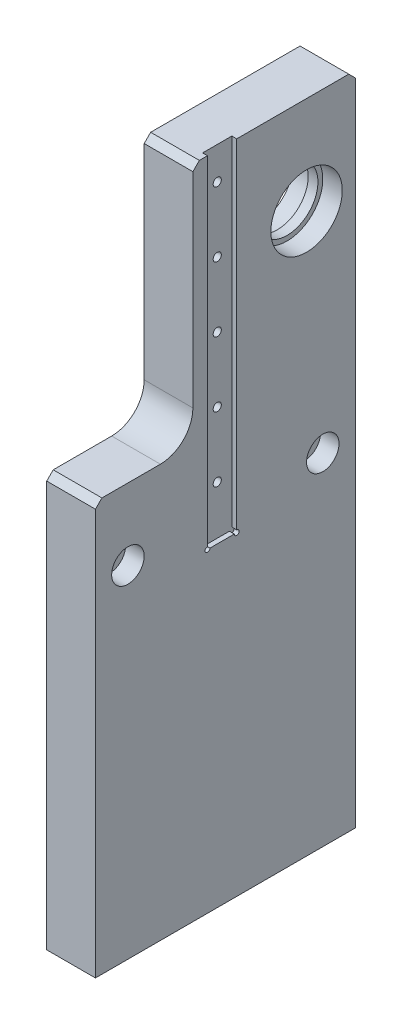
from build123d import *

# Parameters (mm, degrees)
EXTRUDE_1_DEPTH           = 7.5
SKETCH_2_R                = 11
CUT_EXTRUDE_1_DEPTH       = 6
CUT_EXTRUDE_2_REACH       = 111.663
SKETCH_3_R                = 9.5
CUT_EXTRUDE_3_DEPTH       = 1.5
HOLE_WIZARD_M5_1_D        = 4.2
HOLE_WIZARD_M5_1_DEPTH    = 12.4
HOLE_WIZARD_M5_1_TIP      = 1.2618073
HOLE_WIZARD_1_D           = 5.5
HOLE_WIZARD_1_CBORE_D     = 10
HOLE_WIZARD_1_CBORE_DEPTH = 5.7
HOLE_WIZARD_M3_2_D        = 2.5
CUT_EXTRUDE_START         = -6
SKETCH_17_R               = 11
CUT_EXTRUDE_4_DEPTH       = 6
HOLE_WIZARD_M6_1_D        = 5
HOLE_WIZARD_M6_1_DEPTH    = 15
HOLE_WIZARD_M6_1_TIP      = 1.502151548
CHAMFER_1_SIZE            = 2


with BuildPart() as part:
    # 草图1 → 凸台-拉伸1 (new, symmetric)
    with BuildSketch(Plane(origin=(0, 0, 0), x_dir=(0, 0, -1), z_dir=(1, 0, 0))):
        with BuildLine():
            Line((-10, 101), (-10, 36))
            ThreePointArc((-10, 36), (-12.928932188, 28.928932188), (-20, 26))
            Line((-20, 26), (-40, 26))
            Line((-40, 26), (-40, -101))
            Line((-40, -101), (40, -101))
            Line((40, -101), (40, 101))
            Line((40, 101), (-10, 101))
        make_face()
    extrude(amount=EXTRUDE_1_DEPTH, both=True)

    # 草图2 → 切除-拉伸1 (cut)
    with BuildSketch(Plane.ZY.offset(-7.5)):
        with Locations((-25, 71)):
            Circle(SKETCH_2_R)
    extrude(amount=CUT_EXTRUDE_1_DEPTH, mode=Mode.SUBTRACT)

    # 草图3 → 切除-拉伸2 (cut, up to next)
    with BuildSketch(Plane(origin=(-7.5, 0, 0), x_dir=(0, 0, -1), z_dir=(1, 0, 0)), mode=Mode.PRIVATE) as cut_extrude_2_sk1:
        with Locations(Location((25, 71, 0), (0, 0, 180))):
            Circle(SKETCH_3_R)
    cut_extrude_2_tool1 = extrude(cut_extrude_2_sk1.sketch, amount=CUT_EXTRUDE_2_REACH, mode=Mode.PRIVATE) & part.part
    add(cut_extrude_2_tool1.solids().sort_by_distance((-7.5, 71, -25))[0], mode=Mode.SUBTRACT)

    # 草图6 → 切除-拉伸3 (cut)
    with BuildSketch(Plane(origin=(7.5, 0, 0), x_dir=(0, 0, -1), z_dir=(1, 0, 0))):
        with BuildLine():
            Line((-5.5, 101), (3.5, 101))
            Line((3.5, 101), (3.5, -3.25))
            ThreePointArc((3.5, -3.25), (4.030330086, -4.530330086), (2.75, -4))
            Line((2.75, -4), (-4.75, -4))
            ThreePointArc((-4.75, -4), (-6.030330086, -4.530330086), (-5.5, -3.25))
            Line((-5.5, -3.25), (-5.5, 101))
        make_face()
    extrude(amount=-CUT_EXTRUDE_3_DEPTH, mode=Mode.SUBTRACT)

    # M5 螺纹孔1
    with Locations(Plane(origin=(0, -101, 0), x_dir=(-1, 0, 0), z_dir=(0, -1, 0))):
        with Locations((0, 25), (0, -25)):
            Hole(HOLE_WIZARD_M5_1_D / 2, depth=HOLE_WIZARD_M5_1_DEPTH)
            with Locations((0, 0, -(HOLE_WIZARD_M5_1_DEPTH + HOLE_WIZARD_M5_1_TIP / 2))):  # 118° drill point
                Cone(0, HOLE_WIZARD_M5_1_D / 2, HOLE_WIZARD_M5_1_TIP, mode=Mode.SUBTRACT)

    # 打孔尺寸(%根据)内六角圆柱头螺钉的类型1 (through all)
    with Locations(Plane(origin=(7.5, 0, 0), x_dir=(0, 0, -1), z_dir=(1, 0, 0))):
        with Locations((30, 4), (-30, 4)):
            CounterBoreHole(HOLE_WIZARD_1_D / 2, HOLE_WIZARD_1_CBORE_D / 2, HOLE_WIZARD_1_CBORE_DEPTH)

    # M3 螺纹孔2 (through all)
    with Locations(Plane(origin=(6, 0, 0), x_dir=(0, 0, -1), z_dir=(1, 0, 0))):
        with Locations((-1, 91), (-1, 71), (-1, 51), (-1, 31), (-1, 11)):
            Hole(HOLE_WIZARD_M3_2_D / 2)

    # 草图17 → 切除-拉伸4 (cut)
    with BuildSketch(Plane.ZY.offset(7.5).offset(CUT_EXTRUDE_START)):
        with Locations((-25, 71)):
            Circle(SKETCH_17_R)
    extrude(amount=CUT_EXTRUDE_4_DEPTH, mode=Mode.SUBTRACT)

    # M6 螺纹孔1
    with Locations(Plane(origin=(0, 0, -40), x_dir=(-1, 0, 0), z_dir=(0, 0, -1))):
        with Locations((0, 51), (0, 91)):
            Hole(HOLE_WIZARD_M6_1_D / 2, depth=HOLE_WIZARD_M6_1_DEPTH)
            with Locations((0, 0, -(HOLE_WIZARD_M6_1_DEPTH + HOLE_WIZARD_M6_1_TIP / 2))):  # 118° drill point
                Cone(0, HOLE_WIZARD_M6_1_D / 2, HOLE_WIZARD_M6_1_TIP, mode=Mode.SUBTRACT)

    # 倒角1
    chamfer_1_edges = [part.edges().sort_by_distance(p)[0] for p in [
        (0, 26, 40),
        (0, 101, 10),
        (0, 101, -40),
    ]]
    chamfer(chamfer_1_edges, length=CHAMFER_1_SIZE)


solid = part.part
